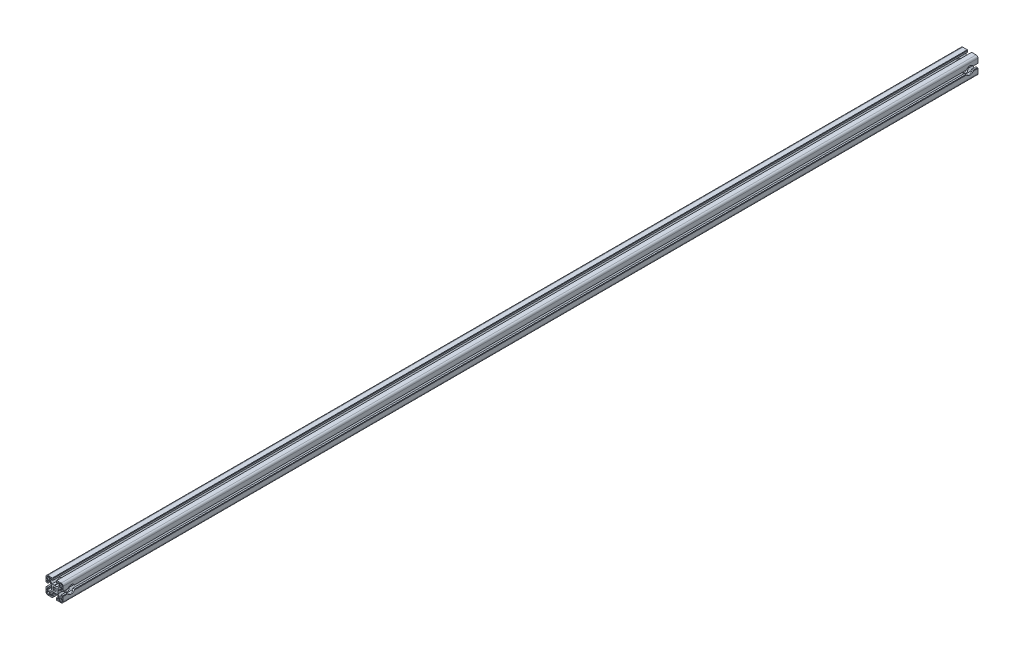
SolidWorks part; units mm, degrees
material "6061 GB/T6892-2006"
ref_plane "前视" through (0, 0, 0) normal (0, 0, 1) x (1, 0, 0)
ref_plane "上视" through (0, 0, 0) normal (0, 1, 0) x (1, 0, 0)
ref_plane "右视" through (0, 0, 0) normal (1, 0, 0) x (0, 0, -1)
sketch "草图1" plane through (0, 0, 0) normal (0, 0, 1) x (1, 0, 0)
  line L0 (-18.9995, -4.1003) -> (-18.9995, -5.1003)
  line L1 (-18.9995, -5.1003) -> (-19.9995, -5.1003)
  line L2 (-19.9995, -5.1003) -> (-19.9995, -15.5003)
  line L3 (-15.4995, -20.0003) -> (-5.0995, -20.0003)
  line L4 (-5.0995, -20.0003) -> (-5.0995, -19.0003)
  line L5 (-5.0995, -19.0003) -> (-4.0995, -19.0003)
  line L6 (-4.0995, -19.0003) -> (-4.0995, -15.5003)
  line L7 (-4.0995, -15.5003) -> (-6.5995, -15.5003)
  line L8 (-6.5995, -15.5003) -> (-6.5995, -16.5003)
  line L9 (-7.5995, -17.5003) -> (-9.7995, -17.5003)
  line L10 (-10.2995, -17.0003) -> (-10.2995, -11.9973)
  line L11 (-10.2995, -11.9973) -> (-5.9025, -7.6003)
  line L12 (-5.9025, -7.6003) -> (-0.5195, -7.6003)
  line L13 (-0.5195, -7.6003) -> (0.0005, -7.3003)
  line L14 (0.0005, -7.3003) -> (0.5195, -7.6003)
  line L15 (0.5195, -7.6003) -> (5.9035, -7.6003)
  line L16 (5.9035, -7.6003) -> (10.3005, -11.9973)
  line L17 (10.3005, -11.9973) -> (10.3005, -17.0003)
  line L18 (9.8005, -17.5003) -> (7.6005, -17.5003)
  line L19 (6.6005, -16.5003) -> (6.6005, -15.5003)
  line L20 (6.6005, -15.5003) -> (4.1005, -15.5003)
  line L21 (4.1005, -15.5003) -> (4.1005, -19.0003)
  line L22 (4.1005, -19.0003) -> (5.1005, -19.0003)
  line L23 (5.1005, -19.0003) -> (5.1005, -20.0003)
  line L24 (5.1005, -20.0003) -> (15.5005, -20.0003)
  line L25 (20.0005, -15.5003) -> (20.0005, -5.1003)
  line L26 (20.0005, -5.1003) -> (19.0005, -5.1003)
  line L27 (19.0005, -5.1003) -> (19.0005, -4.1003)
  line L28 (19.0005, -4.1003) -> (15.5005, -4.1003)
  line L29 (15.5005, -4.1003) -> (15.5005, -6.6003)
  line L30 (15.5005, -6.6003) -> (16.5005, -6.6003)
  line L31 (17.5005, -7.6003) -> (17.5005, -9.8003)
  line L32 (17.0005, -10.3003) -> (11.9975, -10.3003)
  line L33 (11.9975, -10.3003) -> (7.6005, -5.9033)
  line L34 (7.6005, -5.9033) -> (7.6005, -0.5203)
  line L35 (7.6005, -0.5203) -> (7.3005, -0.0003)
  line L36 (7.3005, -0.0003) -> (7.6005, 0.5197)
  line L37 (7.6005, 0.5197) -> (7.6005, 5.9027)
  line L38 (7.6005, 5.9027) -> (11.9975, 10.2997)
  line L39 (11.9975, 10.2997) -> (17.0005, 10.2997)
  line L40 (17.5005, 9.7997) -> (17.5005, 7.5997)
  line L41 (16.5005, 6.5997) -> (15.5005, 6.5997)
  line L42 (15.5005, 6.5997) -> (15.5005, 4.0997)
  line L43 (15.5005, 4.0997) -> (19.0005, 4.0997)
  line L44 (19.0005, 4.0997) -> (19.0005, 5.0997)
  line L45 (19.0005, 5.0997) -> (20.0005, 5.0997)
  line L46 (20.0005, 5.0997) -> (20.0005, 15.4997)
  line L47 (15.5005, 19.9997) -> (5.1005, 19.9997)
  line L48 (5.1005, 19.9997) -> (5.1005, 18.9997)
  line L49 (5.1005, 18.9997) -> (4.1005, 18.9997)
  line L50 (4.1005, 18.9997) -> (4.1005, 15.4997)
  line L51 (4.1005, 15.4997) -> (6.6005, 15.4997)
  line L52 (7.6005, 17.4997) -> (9.8005, 17.4997)
  line L53 (10.3005, 16.9997) -> (10.3005, 11.9967)
  line L54 (10.3005, 11.9967) -> (5.9035, 7.5997)
  line L55 (5.9035, 7.5997) -> (0.5195, 7.5997)
  line L56 (0.5195, 7.5997) -> (0.0005, 7.2997)
  line L57 (0.0005, 7.2997) -> (-0.5195, 7.5997)
  line L58 (-0.5195, 7.5997) -> (-5.9025, 7.5997)
  line L59 (-5.9025, 7.5997) -> (-10.2995, 11.9967)
  line L60 (-10.2995, 11.9967) -> (-10.2995, 16.9997)
  line L61 (-9.7995, 17.4997) -> (-7.5995, 17.4997)
  line L62 (-6.5995, 16.4997) -> (-6.5995, 15.4997)
  line L63 (-6.5995, 15.4997) -> (-4.0995, 15.4997)
  line L64 (-4.0995, 15.4997) -> (-4.0995, 18.9997)
  line L65 (-4.0995, 18.9997) -> (-5.0995, 18.9997)
  line L66 (-5.0995, 18.9997) -> (-5.0995, 19.9997)
  line L67 (-5.0995, 19.9997) -> (-15.4995, 19.9997)
  line L68 (-19.9995, 15.4997) -> (-19.9995, 5.0997)
  line L69 (-19.9995, 5.0997) -> (-18.9995, 5.0997)
  line L70 (-18.9995, 5.0997) -> (-18.9995, 4.0997)
  line L71 (-18.9995, 4.0997) -> (-15.4995, 4.0997)
  line L72 (-15.4995, 4.0997) -> (-15.4995, 6.5997)
  line L73 (-15.4995, 6.5997) -> (-16.4995, 6.5997)
  line L74 (-17.4995, 7.5997) -> (-17.4995, 9.7997)
  line L75 (-16.9995, 10.2997) -> (-11.9965, 10.2997)
  line L76 (-11.9965, 10.2997) -> (-7.5995, 5.9027)
  line L77 (-7.5995, 5.9027) -> (-7.5995, 0.5197)
  line L78 (-7.5995, 0.5197) -> (-7.2995, -0.0003)
  line L79 (-7.2995, -0.0003) -> (-7.5995, -0.5203)
  line L80 (-7.5995, -0.5203) -> (-7.5995, -5.9033)
  line L81 (-7.5995, -5.9033) -> (-11.9965, -10.3003)
  line L82 (-11.9965, -10.3003) -> (-16.9995, -10.3003)
  line L83 (-17.4995, -9.8003) -> (-17.4995, -7.6003)
  line L84 (-16.4995, -6.6003) -> (-15.4995, -6.6003)
  line L85 (-15.4995, -6.6003) -> (-15.4995, -4.1003)
  line L86 (-15.4995, -4.1003) -> (-18.9995, -4.1003)
  line L87 (15.5005, -18.0003) -> (11.8005, -18.0003)
  line L88 (11.8005, -18.0003) -> (11.8005, -11.8003)
  line L89 (11.8005, -11.8003) -> (18.0005, -11.8003)
  line L90 (18.0005, -11.8003) -> (18.0005, -15.5003)
  line L91 (18.0005, 11.7997) -> (11.8005, 11.7997)
  line L92 (11.8005, 11.7997) -> (11.8005, 17.9997)
  line L93 (11.8005, 17.9997) -> (15.5005, 17.9997)
  line L94 (18.0005, 15.4997) -> (18.0005, 11.7997)
  line L95 (-1.8145, -2.8753) -> (-3.0044, -4.0665)
  line L96 (-3.0044, -4.0665) -> (-4.0656, -3.0052)
  line L97 (-4.0656, -3.0052) -> (-2.8745, -1.8153)
  line L98 (-2.8745, 1.8147) -> (-4.0644, 3.0058)
  line L99 (-4.0644, 3.0058) -> (-3.0044, 4.0658)
  line L100 (-3.0044, 4.0658) -> (-1.8145, 2.8747)
  line L101 (1.8145, 2.8747) -> (3.0055, 4.0657)
  line L102 (3.0055, 4.0657) -> (4.0666, 3.0045)
  line L103 (4.0666, 3.0045) -> (2.8755, 1.8147)
  line L104 (2.8755, -1.8153) -> (4.0666, -3.0052)
  line L105 (4.0666, -3.0052) -> (3.0055, -4.0663)
  line L106 (3.0055, -4.0663) -> (1.8145, -2.8753)
  line L107 (-17.9995, -15.5003) -> (-17.9995, -11.8003)
  line L108 (-17.9995, -11.8003) -> (-11.7995, -11.8003)
  line L109 (-11.7995, -11.8003) -> (-11.7995, -18.0003)
  line L110 (-11.7995, -18.0003) -> (-15.4995, -18.0003)
  line L111 (-11.7995, 17.9997) -> (-11.7995, 11.7997)
  line L112 (-11.7995, 11.7997) -> (-17.9995, 11.7997)
  line L113 (-17.9995, 11.7997) -> (-17.9995, 15.4997)
  line L114 (-15.4995, 17.9997) -> (-11.7995, 17.9997)
  arc A0 (-19.9995, -15.5003) -> (-15.4995, -20.0003) centre (-15.4995, -15.5003) ccw
  arc A1 (-6.5995, -16.5003) -> (-7.5995, -17.5003) centre (-7.5995, -16.5003) cw
  arc A2 (-9.7995, -17.5003) -> (-10.2995, -17.0003) centre (-9.7995, -17.0003) cw
  arc A3 (10.3005, -17.0003) -> (9.8005, -17.5003) centre (9.8005, -17.0003) cw
  arc A4 (7.6005, -17.5003) -> (6.6005, -16.5003) centre (7.6005, -16.5003) cw
  arc A5 (15.5005, -20.0003) -> (20.0005, -15.5003) centre (15.5005, -15.5003) ccw
  arc A6 (16.5005, -6.6003) -> (17.5005, -7.6003) centre (16.5005, -7.6003) cw
  arc A7 (17.5005, -9.8003) -> (17.0005, -10.3003) centre (17.0005, -9.8003) cw
  arc A8 (17.0005, 10.2997) -> (17.5005, 9.7997) centre (17.0005, 9.7997) cw
  arc A9 (17.5005, 7.5997) -> (16.5005, 6.5997) centre (16.5005, 7.5997) cw
  arc A10 (20.0005, 15.4997) -> (15.5005, 19.9997) centre (15.5005, 15.4997) ccw
  arc A11 (6.6005, 15.4997) -> (6.6005, 16.4997) centre (7.1003, 15.9997) cw
  arc A12 (6.6005, 16.4997) -> (7.6005, 17.4997) centre (7.6005, 16.4997) cw
  arc A13 (9.8005, 17.4997) -> (10.3005, 16.9997) centre (9.8005, 16.9997) cw
  arc A14 (-10.2995, 16.9997) -> (-9.7995, 17.4997) centre (-9.7995, 16.9997) cw
  arc A15 (-7.5995, 17.4997) -> (-6.5995, 16.4997) centre (-7.5995, 16.4997) cw
  arc A16 (-15.4995, 19.9997) -> (-19.9995, 15.4997) centre (-15.4995, 15.4997) ccw
  arc A17 (-16.4995, 6.5997) -> (-17.4995, 7.5997) centre (-16.4995, 7.5997) cw
  arc A18 (-17.4995, 9.7997) -> (-16.9995, 10.2997) centre (-16.9995, 9.7997) cw
  arc A19 (-16.9995, -10.3003) -> (-17.4995, -9.8003) centre (-16.9995, -9.8003) cw
  arc A20 (-17.4995, -7.6003) -> (-16.4995, -6.6003) centre (-16.4995, -7.6003) cw
  arc A21 (18.0005, -15.5003) -> (15.5005, -18.0003) centre (15.5005, -15.5003) cw
  arc A22 (15.5005, 17.9997) -> (18.0005, 15.4997) centre (15.5005, 15.4997) cw
  arc A23 (-2.8745, -1.8153) -> (-2.8745, 1.8147) centre (0.0005, -0.0003) cw
  arc A24 (-1.8145, 2.8747) -> (1.8145, 2.8747) centre (0, -0.0007) cw
  arc A25 (2.8755, 1.8147) -> (2.8755, -1.8153) centre (0.0005, -0.0003) cw
  arc A26 (1.8145, -2.8753) -> (-1.8145, -2.8753) centre (0, 0) cw
  arc A27 (-15.4995, -18.0003) -> (-17.9995, -15.5003) centre (-15.4995, -15.5003) cw
  arc A28 (-17.9995, 15.4997) -> (-15.4995, 17.9997) centre (-15.4995, 15.4997) cw
extrude "凸台-拉伸1" add sketch "草图1" against normal blind 2144
hole_wizard "Ø19.0 (19) 直径孔1" positions "草图2" profile "草图3" hole size "Ø19.0" standard "GB" end condition through all
sketch "草图2" plane through (20.0005, 0, 0) normal (1, 0, 0) x (0, 0, -1)
  line L0 (2144, -0.0003) -> (0, -0.0003) construction
  point P0 (19, -0.0003)
  point P4 (2125, -0.0003)
  dimension "D1" = 19
  dimension "D2" = 19
sketch "草图3" plane through (20.0005, -0.0003, -19) normal (0, 1, 0) x (0, 0, -1)
  line L0 (0, 0) -> (0, 40)
  line L1 (0, 40) -> (9.5, 40)
  line L2 (9.5, 40) -> (9.5, 0)
  line L5 (9.5, 0) -> (0, 0)
  line L11 (0, -6.35) -> (0, 107.95) construction
  dimension "通孔孔直径" = 19
  dimension "通孔孔深度" = 40
